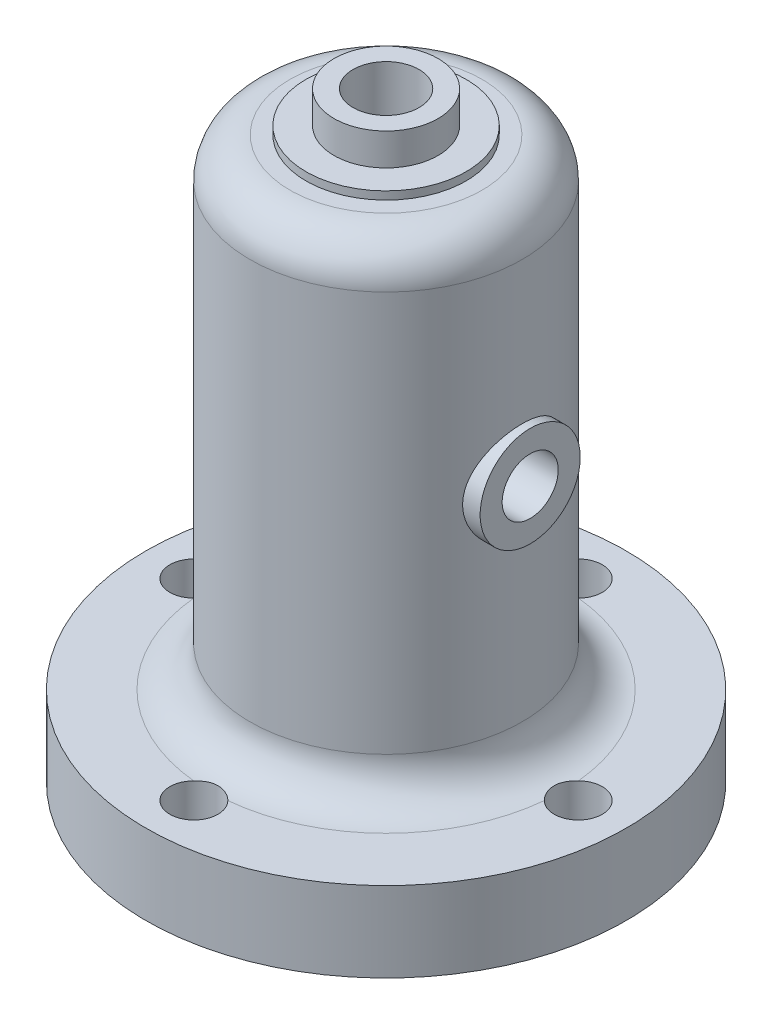
SolidWorks part; units mm, degrees
ref_plane "Front Plane" through (0, 0, 0) normal (0, 0, 1) x (1, 0, 0)
ref_plane "Top Plane" through (0, 0, 0) normal (0, 1, 0) x (1, 0, 0)
ref_plane "Right Plane" through (0, 0, 0) normal (1, 0, 0) x (0, 0, -1)
other "Configuration Table"
sketch "Sketch1" plane through (0, 0, 0) normal (0, 0, 1) x (1, 0, 0)
  line L0 (0, 29.5634) -> (0, -19.533) construction
  line L1 (31.6425, 0) -> (38, 0)
  line L2 (38, 0) -> (38, 2)
  line L3 (38, 2) -> (60, 2)
  line L4 (60, 2) -> (60, 22)
  line L5 (60, 22) -> (44, 22)
  line L6 (34, 32) -> (34, 132)
  line L7 (24, 142) -> (20, 142)
  line L8 (20, 142) -> (20, 144)
  line L9 (20, 144) -> (13, 144)
  line L10 (13, 144) -> (13, 152)
  line L11 (13, 152) -> (0, 152)
  line L12 (0, 152) -> (0, 132)
  line L13 (0, 132) -> (16, 132)
  line L14 (26, 122) -> (26, 32)
  line L15 (26, 32) -> (31.6425, 0)
  arc A0 (34, 132) -> (24, 142) centre (24, 132) ccw
  arc A1 (16, 132) -> (26, 122) centre (16, 122) cw
  arc A2 (44, 22) -> (34, 32) centre (44, 32) cw
  dimension "D15" = 10
  dimension "D16" = 10
  dimension "D1" = 76
  dimension "D2" = 120
  dimension "D3" = 68
  dimension "D4" = 40
  dimension "D5" = 26
  dimension "D6" = 32
  dimension "D7" = 10
  dimension "D8" = 22
  dimension "D9" = 2
  dimension "D10" = 132
  dimension "D11" = 152
  dimension "D12" = 2
  dimension "D13" = 8
  dimension "D14" = 52
revolve "Revolve1" add sketch "Sketch1" angle 360 about L0
cosmetic thread "Cosmetic Thread1" parameters "D2"=20.752
sketch "Sketch2" plane through (0, 0, 0) normal (1, 0, 0) x (0, 0, -1)
  circle A0 centre (0, 84) radius 12.5
  dimension "D1" = 25
  dimension "D2" = 84
extrude "Boss-Extrude1" add sketch "Sketch2" against normal up to next from offset 36
sketch "Sketch3" plane through (36, 0, 0) normal (1, 0, 0) x (0, 0, -1)
  circle A0 centre (0, 84) radius 7
  dimension "D1" = 14
extrude "Cut-Extrude1" cut sketch "Sketch3" against normal up to next
sketch "Sketch4" plane through (0, 22, 0) normal (0, 1, 0) x (1, 0, 0)
  circle A0 centre (0, 0) radius 48 construction
  circle A1 centre (48, 0) radius 6
  circle A2 centre (0, -48) radius 6
  circle A3 centre (-48, 0) radius 6
  circle A4 centre (0, 48) radius 6
  point P14 (0, 0)
  dimension "D1" = 96
  dimension "D2" = 12
  dimension "D3" = 4
extrude "Cut-Extrude2" cut sketch "Sketch4" against normal up to next and the other way up to next
sketch "Sketch6" plane through (0, 152, 0) normal (0, 1, 0) x (1, 0, 0)
  circle A0 centre (0, 0) radius 3.5292
  point P0 (0, 0)
hole_wizard "M18x1.5 Tapped Hole1" positions "Sketch6" profile "Sketch7" tap size "M18x1.5" standard "GB"
sketch "Sketch7" plane through (0, 152, 0) normal (1, 0, 0) x (0, 0, 1)
  line L0 (0, 0) -> (0, 45.4571)
  line L1 (0, 45.4571) -> (8.25, 40.5)
  line L2 (8.25, 40.5) -> (8.25, 0)
  line L5 (8.25, 0) -> (0, 0)
  line L10 (0, 45.4571) -> (-8.25, 40.5) construction
  line L11 (0, -6.35) -> (0, 107.95) construction
  dimension "螺纹孔钻头直径" = 16.5
  dimension "螺纹孔钻头深度" = 40.5
  dimension "导头角度" = 118
cosmetic thread "Cosmetic Thread 1" parameters "D1"=36, "D2"=18
